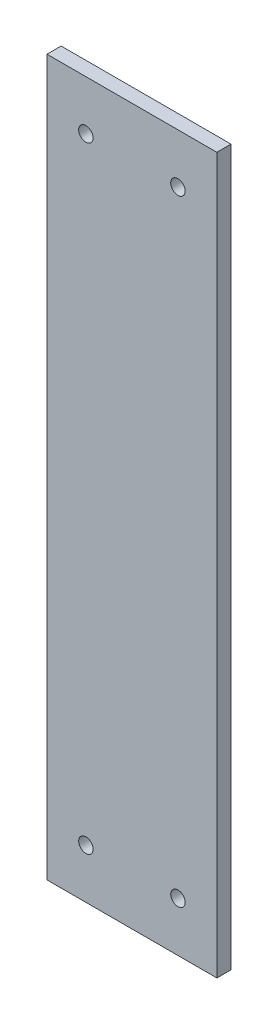
SolidWorks part; units mm, degrees
material "1023 碳钢板 (SS)"
ref_plane "Front Plane" through (0, 0, 0) normal (0, 0, 1) x (1, 0, 0)
ref_plane "Top Plane" through (0, 0, 0) normal (0, 1, 0) x (1, 0, 0)
ref_plane "Right Plane" through (0, 0, 0) normal (1, 0, 0) x (0, 0, -1)
sketch "Sketch1" plane through (0, 0, 0) normal (0, 0, 1) x (1, 0, 0)
  line L1 (60, 252.5) -> (-60, 252.5)
  line L2 (60, 252.5) -> (60, -252.5)
  line L3 (60, -252.5) -> (-60, -252.5)
  line L4 (-60, 252.5) -> (-60, -252.5)
  line L5 (60, 252.5) -> (-60, -252.5) construction
  line L6 (60, -252.5) -> (-60, 252.5) construction
  point P0 (0, 0)
  dimension "D1" = 505
  dimension "D2" = 120
extrude "Boss-Extrude1" add sketch "Sketch1" along normal blind 10 contours L4 L3 L2 L1
sketch "Sketch2" plane through (0, 0, 10) normal (0, 0, 1) x (1, 0, 0)
  line L1 (32.5, -217.5) -> (-32.5, -217.5) construction
  line L2 (32.5, -217.5) -> (32.5, 217.5) construction
  line L3 (32.5, 217.5) -> (-32.5, 217.5) construction
  line L4 (-32.5, -217.5) -> (-32.5, 217.5) construction
  line L5 (32.5, -217.5) -> (-32.5, 217.5) construction
  line L6 (32.5, 217.5) -> (-32.5, -217.5) construction
  circle A0 centre (-32.5, 217.5) radius 4.5
  circle A1 centre (32.5, 217.5) radius 4.5
  circle A2 centre (32.5, -217.5) radius 4.5
  circle A3 centre (-32.5, -217.5) radius 4.5
  point P0 (0, 0)
  dimension "D3" = 9
  dimension "D1" = 65
  dimension "D2" = 435
hole_wizard "M12 Tapped Hole1" positions "Sketch3" profile "Sketch4" tap size "M12" standard "ISO"
sketch "Sketch3" plane through (0, 0, 10) normal (0, 0, 1) x (1, 0, 0)
  point P0 (-32.5, 217.5)
  point P3 (32.5, 217.5)
  point P6 (32.5, -217.5)
  point P9 (-32.5, -217.5)
sketch "Sketch4" plane through (-32.5, 217.5, 10) normal (1, 0, 0) x (0, -1, 0)
  line L0 (0, 0) -> (0, 32.3144)
  line L1 (0, 32.3144) -> (5.1, 29.25)
  line L2 (5.1, 29.25) -> (5.1, 0)
  line L5 (5.1, 0) -> (0, 0)
  line L10 (0, 32.3144) -> (-5.1, 29.25) construction
  line L11 (0, -6.35) -> (0, 107.95) construction
  dimension "螺纹孔钻头直径" = 10.2
  dimension "螺纹孔钻头深度" = 29.25
  dimension "导头角度" = 118
cosmetic thread "Hole Thread Line 1"
cosmetic thread "Hole Thread Line 2"
cosmetic thread "Hole Thread Line 3"
cosmetic thread "Hole Thread Line 4"
